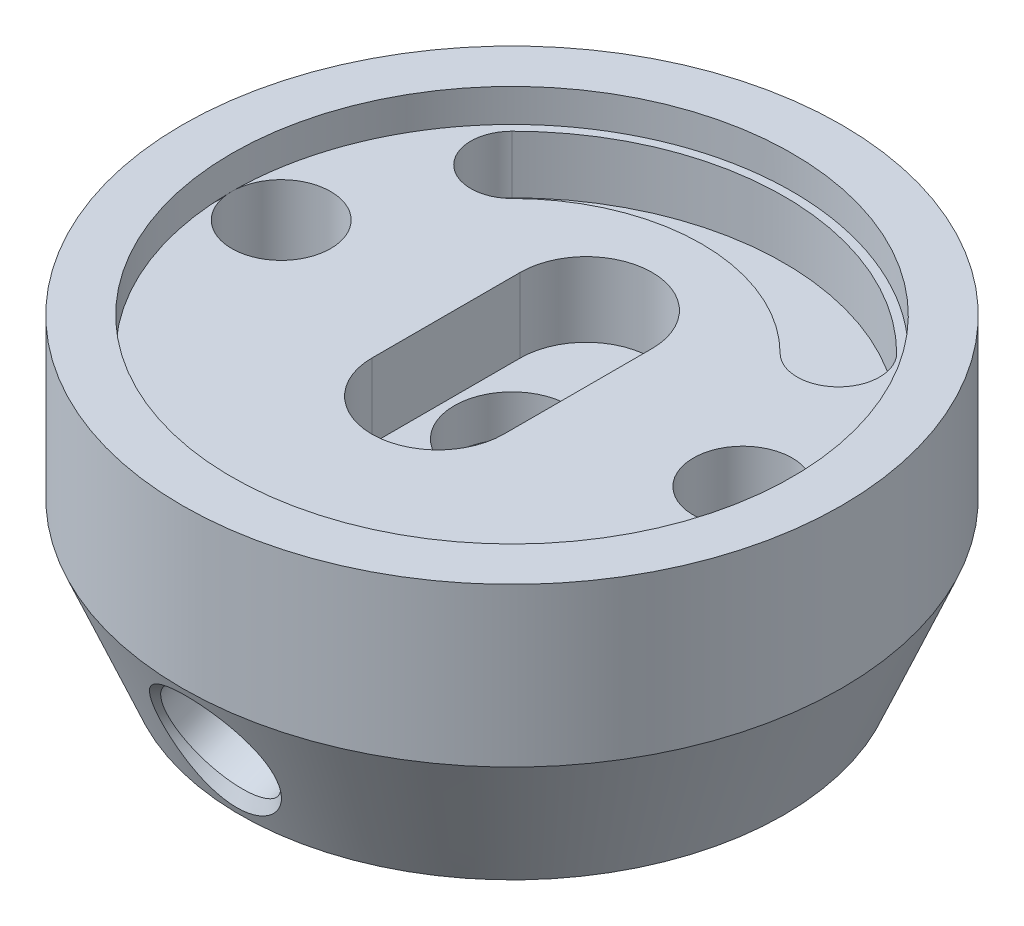
SolidWorks part; units mm, degrees
ref_plane "Front Plane" through (0, 0, 0) normal (0, 0, 1) x (1, 0, 0)
ref_plane "Top Plane" through (0, 0, 0) normal (0, 1, 0) x (1, 0, 0)
ref_plane "Right Plane" through (0, 0, 0) normal (1, 0, 0) x (0, 0, -1)
other "Configuration Table"
sketch "Sketch1" plane through (0, 0, 0) normal (0, 0, 1) x (1, 0, 0)
  line L0 (0, 9.6) -> (0, 0)
  line L1 (0, 0) -> (3.5, -8.4)
  line L2 (3.5, -8.4) -> (20, -8.4)
  line L3 (20, -8.4) -> (20, 9.6) construction
  line L4 (20, 9.6) -> (0, 9.6)
  line L5 (20, 9.6) -> (20, -8.4)
  dimension "D1" = 33
  dimension "D2" = 18
  dimension "D3" = 9.6
  dimension "D4" = 40
revolve "Revolve1" add sketch "Sketch1" angle 360 about L3
sketch "Sketch2" plane through (0, 9.6, 0) normal (0, 1, 0) x (1, 0, 0)
  circle A0 centre (20, 0) radius 17
  dimension "D1" = 34
extrude "Cut-Extrude1" cut sketch "Sketch2" against normal blind 2
sketch "Sketch3" plane through (0, 7.6, 0) normal (0, 1, 0) x (1, 0, 0)
  line L0 (20, 4.5) -> (20, -4.5) construction
  line L1 (24, 4.5) -> (24, -4.5)
  line L2 (16, 4.5) -> (16, -4.5)
  arc A0 (24, 4.5) -> (16, 4.5) centre (20, 4.5) ccw
  arc A1 (16, -4.5) -> (24, -4.5) centre (20, -4.5) ccw
  point P3 (20, 0)
  point P8 (20, 0)
  dimension "D2" = 4
  dimension "D1" = 9
extrude "Cut-Extrude2" cut sketch "Sketch3" against normal blind 4.5
sketch "Sketch4" plane through (0, 7.6, 0) normal (0, 1, 0) x (1, 0, 0)
  line L0 (20, 0) -> (10.1005, 9.8995) construction
  line L1 (20, 0) -> (29.8995, 9.8995) construction
  line L2 (20, 0) -> (20, 20) construction
  arc A0 (10.1005, 9.8995) -> (29.8995, 9.8995) centre (20, 0) cw construction
  arc A1 (31.6673, 11.6673) -> (8.3327, 11.6673) centre (20, 0) ccw
  arc A2 (28.1317, 8.1317) -> (11.8683, 8.1317) centre (20, 0) ccw
  arc A3 (28.1317, 8.1317) -> (31.6673, 11.6673) centre (29.8995, 9.8995) ccw
  arc A4 (8.3327, 11.6673) -> (11.8683, 8.1317) centre (10.1005, 9.8995) ccw
  circle A5 centre (20, 0) radius 20 construction
  point P3 (20, 14)
  point P8 (20, 0)
  dimension "D2" = 2.5
  dimension "D3" = 14
  dimension "D1" = 90
extrude "Cut-Extrude3" cut sketch "Sketch4" against normal blind 3.5
sketch "Sketch5" plane through (0, 7.6, 0) normal (0, 1, 0) x (1, 0, 0)
  line L0 (20, 20) -> (20, -20) construction
  circle A0 centre (6, 0) radius 3
  circle A1 centre (20, 0) radius 20 construction
  circle A2 centre (20, 0) radius 17 construction
  circle A3 centre (34, 0) radius 3
  dimension "D1" = 6
extrude "Cut-Extrude4" cut sketch "Sketch5" against normal blind 11
sketch "Sketch7" plane through (0, -8.4, 0) normal (0, -1, 0) x (1, 0, 0)
  circle A0 centre (20, 0) radius 4.5
  dimension "D1" = 9
extrude "Cut-Extrude5" cut sketch "Sketch7" against normal blind 6
sketch "Sketch8" plane through (0, 3.1, 0) normal (0, 1, 0) x (1, 0, 0)
  circle A0 centre (20, 0) radius 3.5
  point P0 (20, 0)
  dimension "D1" = 7
extrude "Cut-Extrude6" cut sketch "Sketch8" against normal blind 2.5
sketch "Sketch9" plane through (0, 0.6, 0) normal (0, 1, 0) x (1, 0, 0)
  circle A0 centre (20, 0) radius 2.6
  dimension "D1" = 5.2
extrude "Cut-Extrude7" cut sketch "Sketch9" against normal through all
chamfer "Chamfer1" distance 1 angle 45 1 edges at (22.6, -2.4, 0)
sketch "Sketch10" plane through (0, -8.4, 0) normal (0, -1, 0) x (1, 0, 0)
  circle A1 centre (20, 0) radius 6.5
  circle A2 centre (20, 0) radius 14.5
  point P2 (20, 0)
  dimension "D1" = 29
  dimension "D2" = 13
extrude "Cut-Extrude8" cut sketch "Sketch10" against normal blind 0.5
ref_plane "Plane1" through (20, 0, 0) normal (1, 0, 0) x (0, 0, -1)
sketch "Sketch11" plane through (20, 0, 0) normal (1, 0, 0) x (0, 0, -1)
  line L0 (-10.3956, -0.9055) -> (-28.4, -8.4)
  line L1 (-20, 0) -> (20, 0) construction
  line L3 (-20, 0) -> (-16.5, -8.4)
  dimension "D1" = 28.4
  dimension "D2" = 22.6
ref_plane "Plane2" through (0, 2.9164, 1.214) normal (0, 0.9232, 0.3843) x (0, -0.3843, 0.9232)
surface "surface-extrude 1" sketch "Sketch11" parameters "D1"=20
sketch "Sketch12" plane through (0, -7.1006, 17.0414) normal (0, -0.3846, 0.9231) x (1, 0, 0)
  line L0 (20, 7.6923) -> (20, -1.4077) construction
  line L1 (30, 7.6923) -> (10, 7.6923) construction
  line L2 (10, -1.4077) -> (30, -1.4077) construction
  point P7 (20, 3.1423)
hole_wizard "M8 Tapped Hole1" positions "Sketch12" profile "Sketch13" tap size "M8" standard "GB"
sketch "Sketch13" plane through (20, -4.2, 18.25) normal (1, 0, 0) x (0, -0.9231, -0.3846)
  line L0 (0, 0) -> (0, 12.0429)
  line L1 (0, 12.0429) -> (3.4, 10)
  line L2 (3.4, 10) -> (3.4, 0.625)
  line L3 (3.4, 0.625) -> (4.025, 0)
  line L5 (4.025, 0) -> (0, 0)
  line L6 (-3.4, 0.625) -> (-4.025, 0) construction
  line L10 (0, 12.0429) -> (-3.4, 10) construction
  line L11 (0, -6.35) -> (0, 107.95) construction
  dimension "螺纹孔钻头直径" = 6.8
  dimension "螺纹孔钻头深度" = 10
  dimension "近端锥形沉头孔直径" = 8.05
  dimension "近端锥形沉头孔角度" = 90
  dimension "导头角度" = 118
cosmetic thread "hole thread 1" parameters "D1"=7, "D2"=8
